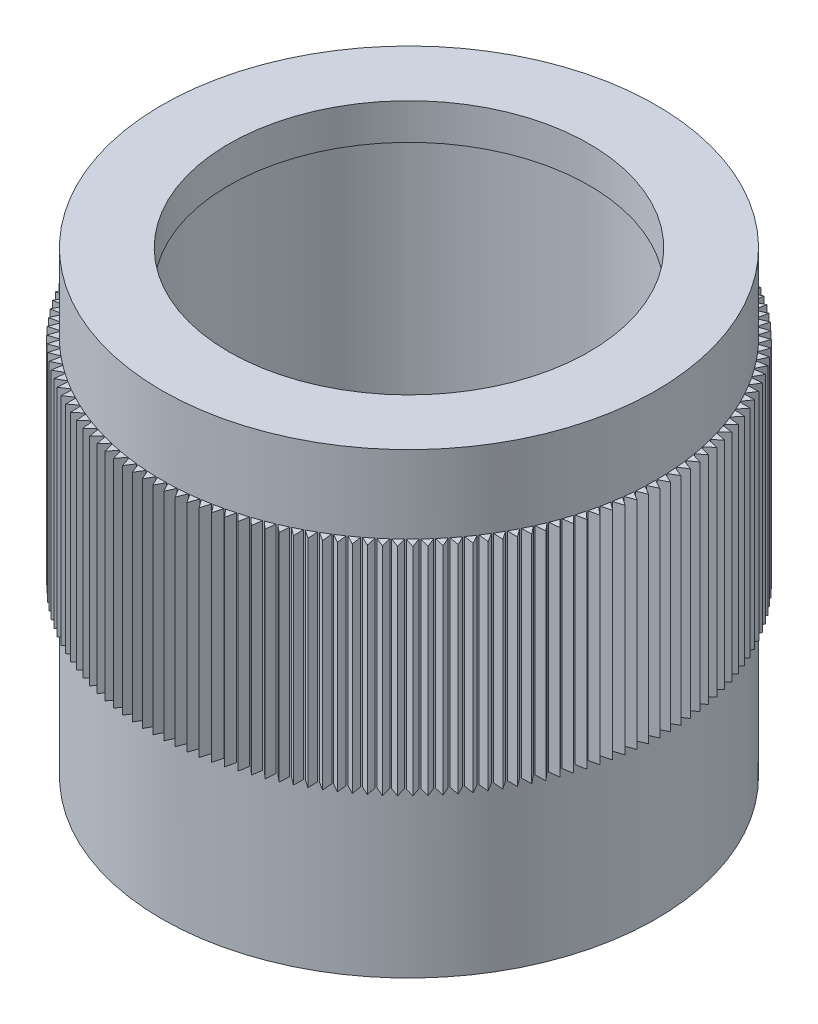
SolidWorks part; units mm, degrees
material "延性铁"
ref_plane "Front Plane" through (0, 0, 0) normal (0, 0, 1) x (1, 0, 0)
ref_plane "Top Plane" through (0, 0, 0) normal (0, 1, 0) x (1, 0, 0)
ref_plane "Right Plane" through (0, 0, 0) normal (1, 0, 0) x (0, 0, -1)
sketch "Sketch1" plane through (0, 0, 0) normal (0, 0, 1) x (1, 0, 0)
  line L0 (0, 15.2542) -> (0, -3.0391) construction
  line L1 (-5, 11.7) -> (-5.25, 11.7)
  line L2 (-5.25, 11.7) -> (-5.25, 0)
  line L3 (-5.25, 0) -> (-6.86, 0)
  line L4 (-6.86, 0) -> (-6.86, 12.7)
  line L5 (-6.86, 12.7) -> (-5, 12.7)
  line L6 (-5, 12.7) -> (-5, 11.7)
  dimension "D1" = 13.72
  dimension "D2" = 10.5
  dimension "D3" = 1
  dimension "D4" = 12.7
  dimension "D5" = 10
revolve "Revolve1" add sketch "Sketch1" angle 360 about L0
cosmetic thread "Cosmetic Thread2" parameters "D1"=8, "D2"=10.7
ref_plane "Plane1" through (0, 10.55, 0) normal (0, 1, 0) x (-1, 0, 0)
sketch "Sketch2" plane through (0, 10.55, 0) normal (0, 1, 0) x (-1, 0, 0)
  line L0 (0, -1.1989) -> (0, 9.5046) construction
  line L1 (-0.125, 6.8589) -> (0, 7.11)
  line L2 (0, 7.11) -> (0.125, 6.8589)
  line L3 (0.1623, 6.8581) -> (0.2977, 7.1038)
  line L4 (0.2977, 7.1038) -> (0.4121, 6.8476)
  line L5 (0.4494, 6.8453) -> (0.5949, 7.0851)
  line L6 (0.5949, 7.0851) -> (0.6985, 6.8243)
  line L7 (0.7356, 6.8204) -> (0.8911, 7.0539)
  line L8 (0.8911, 7.0539) -> (0.9837, 6.7891)
  line L9 (1.0206, 6.7837) -> (1.1857, 7.0104)
  line L10 (1.1857, 7.0104) -> (1.2671, 6.742)
  line L11 (1.3038, 6.735) -> (1.4783, 6.9546)
  line L12 (1.4783, 6.9546) -> (1.5483, 6.683)
  line L13 (1.5847, 6.6745) -> (1.7682, 6.8866)
  line L14 (1.7682, 6.8866) -> (1.8268, 6.6123)
  line L15 (1.8628, 6.6023) -> (2.055, 6.8065)
  line L16 (2.055, 6.8065) -> (2.1021, 6.53)
  line L17 (2.1376, 6.5185) -> (2.3382, 6.7145)
  line L18 (2.3382, 6.7145) -> (2.3737, 6.4362)
  line L19 (2.4087, 6.4232) -> (2.6174, 6.6107)
  line L20 (2.6174, 6.6107) -> (2.6411, 6.3312)
  line L21 (2.6756, 6.3167) -> (2.8919, 6.4953)
  line L22 (2.8919, 6.4953) -> (2.9039, 6.215)
  line L23 (2.9377, 6.1991) -> (3.1614, 6.3685)
  line L24 (3.1614, 6.3685) -> (3.1617, 6.088)
  line L25 (3.1947, 6.0707) -> (3.4253, 6.2305)
  line L26 (3.4253, 6.2305) -> (3.4138, 5.9502)
  line L27 (3.4462, 5.9316) -> (3.6832, 6.0816)
  line L28 (3.6832, 6.0816) -> (3.66, 5.8021)
  line L29 (3.6915, 5.7821) -> (3.9346, 5.9221)
  line L30 (3.9346, 5.9221) -> (3.8998, 5.6437)
  line L31 (3.9304, 5.6224) -> (4.1792, 5.7521)
  line L32 (4.1792, 5.7521) -> (4.1327, 5.4755)
  line L33 (4.1624, 5.4529) -> (4.4164, 5.5721)
  line L34 (4.4164, 5.5721) -> (4.3583, 5.2976)
  line L35 (4.3871, 5.2738) -> (4.6458, 5.3822)
  line L36 (4.6458, 5.3822) -> (4.5763, 5.1104)
  line L37 (4.6041, 5.0855) -> (4.8671, 5.183)
  line L38 (4.8671, 5.183) -> (4.7863, 4.9143)
  line L39 (4.813, 4.8882) -> (5.0799, 4.9746)
  line L40 (5.0799, 4.9746) -> (4.9879, 4.7096)
  line L41 (5.0135, 4.6824) -> (5.2838, 4.7575)
  line L42 (5.2838, 4.7575) -> (5.1808, 4.4966)
  line L43 (5.2052, 4.4683) -> (5.4783, 4.5321)
  line L44 (5.4783, 4.5321) -> (5.3645, 4.2757)
  line L45 (5.3877, 4.2464) -> (5.6633, 4.2987)
  line L46 (5.6633, 4.2987) -> (5.5389, 4.0473)
  line L47 (5.5608, 4.0171) -> (5.8384, 4.0578)
  line L48 (5.8384, 4.0578) -> (5.7035, 3.8118)
  line L49 (5.7241, 3.7807) -> (6.0032, 3.8097)
  line L50 (6.0032, 3.8097) -> (5.8581, 3.5696)
  line L51 (5.8774, 3.5377) -> (6.1574, 3.555)
  line L52 (6.1574, 3.555) -> (6.0024, 3.3212)
  line L53 (6.0204, 3.2885) -> (6.3009, 3.294)
  line L54 (6.3009, 3.294) -> (6.1363, 3.0669)
  line L55 (6.1529, 3.0335) -> (6.4333, 3.0273)
  line L56 (6.4333, 3.0273) -> (6.2593, 2.8073)
  line L57 (6.2745, 2.7731) -> (6.5544, 2.7552)
  line L58 (6.5544, 2.7552) -> (6.3714, 2.5427)
  line L59 (6.3851, 2.508) -> (6.6641, 2.4783)
  line L60 (6.6641, 2.4783) -> (6.4723, 2.2736)
  line L61 (6.4845, 2.2384) -> (6.762, 2.1971)
  line L62 (6.762, 2.1971) -> (6.5618, 2.0006)
  line L63 (6.5726, 1.9649) -> (6.8481, 1.912)
  line L64 (6.8481, 1.912) -> (6.6398, 1.7241)
  line L65 (6.6491, 1.6879) -> (6.9221, 1.6236)
  line L66 (6.9221, 1.6236) -> (6.7062, 1.4445)
  line L67 (6.7139, 1.408) -> (6.9841, 1.3323)
  line L68 (6.9841, 1.3323) -> (6.7608, 1.1624)
  line L69 (6.767, 1.1256) -> (7.0337, 1.0387)
  line L70 (7.0337, 1.0387) -> (6.8035, 0.8783)
  line L71 (6.8082, 0.8413) -> (7.0711, 0.7432)
  line L72 (7.0711, 0.7432) -> (6.8344, 0.5926)
  line L73 (6.8375, 0.5554) -> (7.096, 0.4464)
  line L74 (7.096, 0.4464) -> (6.8532, 0.3059)
  line L75 (6.8547, 0.2686) -> (7.1084, 0.1489)
  line L76 (7.1084, 0.1489) -> (6.86, 0.0187)
  line L77 (6.86, -0.0187) -> (7.1084, -0.1489)
  line L78 (7.1084, -0.1489) -> (6.8547, -0.2686)
  line L79 (6.8532, -0.3059) -> (7.096, -0.4464)
  line L80 (7.096, -0.4464) -> (6.8375, -0.5554)
  line L81 (6.8344, -0.5926) -> (7.0711, -0.7432)
  line L82 (7.0711, -0.7432) -> (6.8082, -0.8413)
  line L83 (6.8035, -0.8783) -> (7.0337, -1.0387)
  line L84 (7.0337, -1.0387) -> (6.767, -1.1256)
  line L85 (6.7608, -1.1624) -> (6.9841, -1.3323)
  line L86 (6.9841, -1.3323) -> (6.7139, -1.408)
  line L87 (6.7062, -1.4445) -> (6.9221, -1.6236)
  line L88 (6.9221, -1.6236) -> (6.6491, -1.6879)
  line L89 (6.6398, -1.7241) -> (6.8481, -1.912)
  line L90 (6.8481, -1.912) -> (6.5726, -1.9649)
  line L91 (6.5618, -2.0006) -> (6.762, -2.1971)
  line L92 (6.762, -2.1971) -> (6.4845, -2.2384)
  line L93 (6.4723, -2.2736) -> (6.6641, -2.4783)
  line L94 (6.6641, -2.4783) -> (6.3851, -2.508)
  line L95 (6.3714, -2.5427) -> (6.5544, -2.7552)
  line L96 (6.5544, -2.7552) -> (6.2745, -2.7731)
  line L97 (6.2593, -2.8073) -> (6.4333, -3.0273)
  line L98 (6.4333, -3.0273) -> (6.1529, -3.0335)
  line L99 (6.1363, -3.0669) -> (6.3009, -3.294)
  line L100 (6.3009, -3.294) -> (6.0204, -3.2885)
  line L101 (6.0024, -3.3212) -> (6.1574, -3.555)
  line L102 (6.1574, -3.555) -> (5.8774, -3.5377)
  line L103 (5.8581, -3.5696) -> (6.0032, -3.8097)
  line L104 (6.0032, -3.8097) -> (5.7241, -3.7807)
  line L105 (5.7035, -3.8118) -> (5.8384, -4.0578)
  line L106 (5.8384, -4.0578) -> (5.5608, -4.0171)
  line L107 (5.5389, -4.0473) -> (5.6633, -4.2987)
  line L108 (5.6633, -4.2987) -> (5.3877, -4.2464)
  line L109 (5.3645, -4.2757) -> (5.4783, -4.5321)
  line L110 (5.4783, -4.5321) -> (5.2052, -4.4683)
  line L111 (5.1808, -4.4966) -> (5.2838, -4.7575)
  line L112 (5.2838, -4.7575) -> (5.0135, -4.6824)
  line L113 (4.9879, -4.7096) -> (5.0799, -4.9746)
  line L114 (5.0799, -4.9746) -> (4.813, -4.8882)
  line L115 (4.7863, -4.9143) -> (4.8671, -5.183)
  line L116 (4.8671, -5.183) -> (4.6041, -5.0855)
  line L117 (4.5763, -5.1104) -> (4.6458, -5.3822)
  line L118 (4.6458, -5.3822) -> (4.3871, -5.2738)
  line L119 (4.3583, -5.2976) -> (4.4164, -5.5721)
  line L120 (4.4164, -5.5721) -> (4.1624, -5.4529)
  line L121 (4.1327, -5.4755) -> (4.1792, -5.7521)
  line L122 (4.1792, -5.7521) -> (3.9304, -5.6224)
  line L123 (3.8998, -5.6437) -> (3.9346, -5.9221)
  line L124 (3.9346, -5.9221) -> (3.6915, -5.7821)
  line L125 (3.66, -5.8021) -> (3.6832, -6.0816)
  line L126 (3.6832, -6.0816) -> (3.4462, -5.9316)
  line L127 (3.4138, -5.9502) -> (3.4253, -6.2305)
  line L128 (3.4253, -6.2305) -> (3.1947, -6.0707)
  line L129 (3.1617, -6.088) -> (3.1614, -6.3685)
  line L130 (3.1614, -6.3685) -> (2.9377, -6.1991)
  line L131 (2.9039, -6.215) -> (2.8919, -6.4953)
  line L132 (2.8919, -6.4953) -> (2.6756, -6.3167)
  line L133 (2.6411, -6.3312) -> (2.6174, -6.6107)
  line L134 (2.6174, -6.6107) -> (2.4087, -6.4232)
  line L135 (2.3737, -6.4362) -> (2.3382, -6.7145)
  line L136 (2.3382, -6.7145) -> (2.1376, -6.5185)
  line L137 (2.1021, -6.53) -> (2.055, -6.8065)
  line L138 (2.055, -6.8065) -> (1.8628, -6.6023)
  line L139 (1.8268, -6.6123) -> (1.7682, -6.8866)
  line L140 (1.7682, -6.8866) -> (1.5847, -6.6745)
  line L141 (1.5483, -6.683) -> (1.4783, -6.9546)
  line L142 (1.4783, -6.9546) -> (1.3038, -6.735)
  line L143 (1.2671, -6.742) -> (1.1857, -7.0104)
  line L144 (1.1857, -7.0104) -> (1.0206, -6.7837)
  line L145 (0.9837, -6.7891) -> (0.8911, -7.0539)
  line L146 (0.8911, -7.0539) -> (0.7356, -6.8204)
  line L147 (0.6985, -6.8243) -> (0.5949, -7.0851)
  line L148 (0.5949, -7.0851) -> (0.4494, -6.8453)
  line L149 (0.4121, -6.8476) -> (0.2977, -7.1038)
  line L150 (0.2977, -7.1038) -> (0.1623, -6.8581)
  line L151 (0.125, -6.8589) -> (0, -7.11)
  line L152 (0, -7.11) -> (-0.125, -6.8589)
  line L153 (-0.1623, -6.8581) -> (-0.2977, -7.1038)
  line L154 (-0.2977, -7.1038) -> (-0.4121, -6.8476)
  line L155 (-0.4494, -6.8453) -> (-0.5949, -7.0851)
  line L156 (-0.5949, -7.0851) -> (-0.6985, -6.8243)
  line L157 (-0.7356, -6.8204) -> (-0.8911, -7.0539)
  line L158 (-0.8911, -7.0539) -> (-0.9837, -6.7891)
  line L159 (-1.0206, -6.7837) -> (-1.1857, -7.0104)
  line L160 (-1.1857, -7.0104) -> (-1.2671, -6.742)
  line L161 (-1.3038, -6.735) -> (-1.4783, -6.9546)
  line L162 (-1.4783, -6.9546) -> (-1.5483, -6.683)
  line L163 (-1.5847, -6.6745) -> (-1.7682, -6.8866)
  line L164 (-1.7682, -6.8866) -> (-1.8268, -6.6123)
  line L165 (-1.8628, -6.6023) -> (-2.055, -6.8065)
  line L166 (-2.055, -6.8065) -> (-2.1021, -6.53)
  line L167 (-2.1376, -6.5185) -> (-2.3382, -6.7145)
  line L168 (-2.3382, -6.7145) -> (-2.3737, -6.4362)
  line L169 (-2.4087, -6.4232) -> (-2.6174, -6.6107)
  line L170 (-2.6174, -6.6107) -> (-2.6411, -6.3312)
  line L171 (-2.6756, -6.3167) -> (-2.8919, -6.4953)
  line L172 (-2.8919, -6.4953) -> (-2.9039, -6.215)
  line L173 (-2.9377, -6.1991) -> (-3.1614, -6.3685)
  line L174 (-3.1614, -6.3685) -> (-3.1617, -6.088)
  line L175 (-3.1947, -6.0707) -> (-3.4253, -6.2305)
  line L176 (-3.4253, -6.2305) -> (-3.4138, -5.9502)
  line L177 (-3.4462, -5.9316) -> (-3.6832, -6.0816)
  line L178 (-3.6832, -6.0816) -> (-3.66, -5.8021)
  line L179 (-3.6915, -5.7821) -> (-3.9346, -5.9221)
  line L180 (-3.9346, -5.9221) -> (-3.8998, -5.6437)
  line L181 (-3.9304, -5.6224) -> (-4.1792, -5.7521)
  line L182 (-4.1792, -5.7521) -> (-4.1327, -5.4755)
  line L183 (-4.1624, -5.4529) -> (-4.4164, -5.5721)
  line L184 (-4.4164, -5.5721) -> (-4.3583, -5.2976)
  line L185 (-4.3871, -5.2738) -> (-4.6458, -5.3822)
  line L186 (-4.6458, -5.3822) -> (-4.5763, -5.1104)
  line L187 (-4.6041, -5.0855) -> (-4.8671, -5.183)
  line L188 (-4.8671, -5.183) -> (-4.7863, -4.9143)
  line L189 (-4.813, -4.8882) -> (-5.0799, -4.9746)
  line L190 (-5.0799, -4.9746) -> (-4.9879, -4.7096)
  line L191 (-5.0135, -4.6824) -> (-5.2838, -4.7575)
  line L192 (-5.2838, -4.7575) -> (-5.1808, -4.4966)
  line L193 (-5.2052, -4.4683) -> (-5.4783, -4.5321)
  line L194 (-5.4783, -4.5321) -> (-5.3645, -4.2757)
  line L195 (-5.3877, -4.2464) -> (-5.6633, -4.2987)
  line L196 (-5.6633, -4.2987) -> (-5.5389, -4.0473)
  line L197 (-5.5608, -4.0171) -> (-5.8384, -4.0578)
  line L198 (-5.8384, -4.0578) -> (-5.7035, -3.8118)
  line L199 (-5.7241, -3.7807) -> (-6.0032, -3.8097)
  line L200 (-6.0032, -3.8097) -> (-5.8581, -3.5696)
  line L201 (-5.8774, -3.5377) -> (-6.1574, -3.555)
  line L202 (-6.1574, -3.555) -> (-6.0024, -3.3212)
  line L203 (-6.0204, -3.2885) -> (-6.3009, -3.294)
  line L204 (-6.3009, -3.294) -> (-6.1363, -3.0669)
  line L205 (-6.1529, -3.0335) -> (-6.4333, -3.0273)
  line L206 (-6.4333, -3.0273) -> (-6.2593, -2.8073)
  line L207 (-6.2745, -2.7731) -> (-6.5544, -2.7552)
  line L208 (-6.5544, -2.7552) -> (-6.3714, -2.5427)
  line L209 (-6.3851, -2.508) -> (-6.6641, -2.4783)
  line L210 (-6.6641, -2.4783) -> (-6.4723, -2.2736)
  line L211 (-6.4845, -2.2384) -> (-6.762, -2.1971)
  line L212 (-6.762, -2.1971) -> (-6.5618, -2.0006)
  line L213 (-6.5726, -1.9649) -> (-6.8481, -1.912)
  line L214 (-6.8481, -1.912) -> (-6.6398, -1.7241)
  line L215 (-6.6491, -1.6879) -> (-6.9221, -1.6236)
  line L216 (-6.9221, -1.6236) -> (-6.7062, -1.4445)
  line L217 (-6.7139, -1.408) -> (-6.9841, -1.3323)
  line L218 (-6.9841, -1.3323) -> (-6.7608, -1.1624)
  line L219 (-6.767, -1.1256) -> (-7.0337, -1.0387)
  line L220 (-7.0337, -1.0387) -> (-6.8035, -0.8783)
  line L221 (-6.8082, -0.8413) -> (-7.0711, -0.7432)
  line L222 (-7.0711, -0.7432) -> (-6.8344, -0.5926)
  line L223 (-6.8375, -0.5554) -> (-7.096, -0.4464)
  line L224 (-7.096, -0.4464) -> (-6.8532, -0.3059)
  line L225 (-6.8547, -0.2686) -> (-7.1084, -0.1489)
  line L226 (-7.1084, -0.1489) -> (-6.86, -0.0187)
  line L227 (-6.86, 0.0187) -> (-7.1084, 0.1489)
  line L228 (-7.1084, 0.1489) -> (-6.8547, 0.2686)
  line L229 (-6.8532, 0.3059) -> (-7.096, 0.4464)
  line L230 (-7.096, 0.4464) -> (-6.8375, 0.5554)
  line L231 (-6.8344, 0.5926) -> (-7.0711, 0.7432)
  line L232 (-7.0711, 0.7432) -> (-6.8082, 0.8413)
  line L233 (-6.8035, 0.8783) -> (-7.0337, 1.0387)
  line L234 (-7.0337, 1.0387) -> (-6.767, 1.1256)
  line L235 (-6.7608, 1.1624) -> (-6.9841, 1.3323)
  line L236 (-6.9841, 1.3323) -> (-6.7139, 1.408)
  line L237 (-6.7062, 1.4445) -> (-6.9221, 1.6236)
  line L238 (-6.9221, 1.6236) -> (-6.6491, 1.6879)
  line L239 (-6.6398, 1.7241) -> (-6.8481, 1.912)
  line L240 (-6.8481, 1.912) -> (-6.5726, 1.9649)
  line L241 (-6.5618, 2.0006) -> (-6.762, 2.1971)
  line L242 (-6.762, 2.1971) -> (-6.4845, 2.2384)
  line L243 (-6.4723, 2.2736) -> (-6.6641, 2.4783)
  line L244 (-6.6641, 2.4783) -> (-6.3851, 2.508)
  line L245 (-6.3714, 2.5427) -> (-6.5544, 2.7552)
  line L246 (-6.5544, 2.7552) -> (-6.2745, 2.7731)
  line L247 (-6.2593, 2.8073) -> (-6.4333, 3.0273)
  line L248 (-6.4333, 3.0273) -> (-6.1529, 3.0335)
  line L249 (-6.1363, 3.0669) -> (-6.3009, 3.294)
  line L250 (-6.3009, 3.294) -> (-6.0204, 3.2885)
  line L251 (-6.0024, 3.3212) -> (-6.1574, 3.555)
  line L252 (-6.1574, 3.555) -> (-5.8774, 3.5377)
  line L253 (-5.8581, 3.5696) -> (-6.0032, 3.8097)
  line L254 (-6.0032, 3.8097) -> (-5.7241, 3.7807)
  line L255 (-5.7035, 3.8118) -> (-5.8384, 4.0578)
  line L256 (-5.8384, 4.0578) -> (-5.5608, 4.0171)
  line L257 (-5.5389, 4.0473) -> (-5.6633, 4.2987)
  line L258 (-5.6633, 4.2987) -> (-5.3877, 4.2464)
  line L259 (-5.3645, 4.2757) -> (-5.4783, 4.5321)
  line L260 (-5.4783, 4.5321) -> (-5.2052, 4.4683)
  line L261 (-5.1808, 4.4966) -> (-5.2838, 4.7575)
  line L262 (-5.2838, 4.7575) -> (-5.0135, 4.6824)
  line L263 (-4.9879, 4.7096) -> (-5.0799, 4.9746)
  line L264 (-5.0799, 4.9746) -> (-4.813, 4.8882)
  line L265 (-4.7863, 4.9143) -> (-4.8671, 5.183)
  line L266 (-4.8671, 5.183) -> (-4.6041, 5.0855)
  line L267 (-4.5763, 5.1104) -> (-4.6458, 5.3822)
  line L268 (-4.6458, 5.3822) -> (-4.3871, 5.2738)
  line L269 (-4.3583, 5.2976) -> (-4.4164, 5.5721)
  line L270 (-4.4164, 5.5721) -> (-4.1624, 5.4529)
  line L271 (-4.1327, 5.4755) -> (-4.1792, 5.7521)
  line L272 (-4.1792, 5.7521) -> (-3.9304, 5.6224)
  line L273 (-3.8998, 5.6437) -> (-3.9346, 5.9221)
  line L274 (-3.9346, 5.9221) -> (-3.6915, 5.7821)
  line L275 (-3.66, 5.8021) -> (-3.6832, 6.0816)
  line L276 (-3.6832, 6.0816) -> (-3.4462, 5.9316)
  line L277 (-3.4138, 5.9502) -> (-3.4253, 6.2305)
  line L278 (-3.4253, 6.2305) -> (-3.1947, 6.0707)
  line L279 (-3.1617, 6.088) -> (-3.1614, 6.3685)
  line L280 (-3.1614, 6.3685) -> (-2.9377, 6.1991)
  line L281 (-2.9039, 6.215) -> (-2.8919, 6.4953)
  line L282 (-2.8919, 6.4953) -> (-2.6756, 6.3167)
  line L283 (-2.6411, 6.3312) -> (-2.6174, 6.6107)
  line L284 (-2.6174, 6.6107) -> (-2.4087, 6.4232)
  line L285 (-2.3737, 6.4362) -> (-2.3382, 6.7145)
  line L286 (-2.3382, 6.7145) -> (-2.1376, 6.5185)
  line L287 (-2.1021, 6.53) -> (-2.055, 6.8065)
  line L288 (-2.055, 6.8065) -> (-1.8628, 6.6023)
  line L289 (-1.8268, 6.6123) -> (-1.7682, 6.8866)
  line L290 (-1.7682, 6.8866) -> (-1.5847, 6.6745)
  line L291 (-1.5483, 6.683) -> (-1.4783, 6.9546)
  line L292 (-1.4783, 6.9546) -> (-1.3038, 6.735)
  line L293 (-1.2671, 6.742) -> (-1.1857, 7.0104)
  line L294 (-1.1857, 7.0104) -> (-1.0206, 6.7837)
  line L295 (-0.9837, 6.7891) -> (-0.8911, 7.0539)
  line L296 (-0.8911, 7.0539) -> (-0.7356, 6.8204)
  line L297 (-0.6985, 6.8243) -> (-0.5949, 7.0851)
  line L298 (-0.5949, 7.0851) -> (-0.4494, 6.8453)
  line L299 (-0.4121, 6.8476) -> (-0.2977, 7.1038)
  line L300 (-0.2977, 7.1038) -> (-0.1623, 6.8581)
  circle A0 centre (0, 0) radius 6.86 construction
  arc A1 (0.125, 6.8589) -> (-0.125, 6.8589) centre (0, 0) ccw
  arc A2 (0.4121, 6.8476) -> (0.1623, 6.8581) centre (0, 0) ccw
  arc A3 (0.6985, 6.8243) -> (0.4494, 6.8453) centre (0, 0) ccw
  arc A4 (0.9837, 6.7891) -> (0.7356, 6.8204) centre (0, 0) ccw
  arc A5 (1.2671, 6.742) -> (1.0206, 6.7837) centre (0, 0) ccw
  arc A6 (1.5483, 6.683) -> (1.3038, 6.735) centre (0, 0) ccw
  arc A7 (1.8268, 6.6123) -> (1.5847, 6.6745) centre (0, 0) ccw
  arc A8 (2.1021, 6.53) -> (1.8628, 6.6023) centre (0, 0) ccw
  arc A9 (2.3737, 6.4362) -> (2.1376, 6.5185) centre (0, 0) ccw
  arc A10 (2.6411, 6.3312) -> (2.4087, 6.4232) centre (0, 0) ccw
  arc A11 (2.9039, 6.215) -> (2.6756, 6.3167) centre (0, 0) ccw
  arc A12 (3.1617, 6.088) -> (2.9377, 6.1991) centre (0, 0) ccw
  arc A13 (3.4138, 5.9502) -> (3.1947, 6.0707) centre (0, 0) ccw
  arc A14 (3.66, 5.8021) -> (3.4462, 5.9316) centre (0, 0) ccw
  arc A15 (3.8998, 5.6437) -> (3.6915, 5.7821) centre (0, 0) ccw
  arc A16 (4.1327, 5.4755) -> (3.9304, 5.6224) centre (0, 0) ccw
  arc A17 (4.3583, 5.2976) -> (4.1624, 5.4529) centre (0, 0) ccw
  arc A18 (4.5763, 5.1104) -> (4.3871, 5.2738) centre (0, 0) ccw
  arc A19 (4.7863, 4.9143) -> (4.6041, 5.0855) centre (0, 0) ccw
  arc A20 (4.9879, 4.7096) -> (4.813, 4.8882) centre (0, 0) ccw
  arc A21 (5.1808, 4.4966) -> (5.0135, 4.6824) centre (0, 0) ccw
  arc A22 (5.3645, 4.2757) -> (5.2052, 4.4683) centre (0, 0) ccw
  arc A23 (5.5389, 4.0473) -> (5.3877, 4.2464) centre (0, 0) ccw
  arc A24 (5.7035, 3.8118) -> (5.5608, 4.0171) centre (0, 0) ccw
  arc A25 (5.8581, 3.5696) -> (5.7241, 3.7807) centre (0, 0) ccw
  arc A26 (6.0024, 3.3212) -> (5.8774, 3.5377) centre (0, 0) ccw
  arc A27 (6.1363, 3.0669) -> (6.0204, 3.2885) centre (0, 0) ccw
  arc A28 (6.2593, 2.8073) -> (6.1529, 3.0335) centre (0, 0) ccw
  arc A29 (6.3714, 2.5427) -> (6.2745, 2.7731) centre (0, 0) ccw
  arc A30 (6.4723, 2.2736) -> (6.3851, 2.508) centre (0, 0) ccw
  arc A31 (6.5618, 2.0006) -> (6.4845, 2.2384) centre (0, 0) ccw
  arc A32 (6.6398, 1.7241) -> (6.5726, 1.9649) centre (0, 0) ccw
  arc A33 (6.7062, 1.4445) -> (6.6491, 1.6879) centre (0, 0) ccw
  arc A34 (6.7608, 1.1624) -> (6.7139, 1.408) centre (0, 0) ccw
  arc A35 (6.8035, 0.8783) -> (6.767, 1.1256) centre (0, 0) ccw
  arc A36 (6.8344, 0.5926) -> (6.8082, 0.8413) centre (0, 0) ccw
  arc A37 (6.8532, 0.3059) -> (6.8375, 0.5554) centre (0, 0) ccw
  arc A38 (6.86, 0.0187) -> (6.8547, 0.2686) centre (0, 0) ccw
  arc A39 (6.8547, -0.2686) -> (6.86, -0.0187) centre (0, 0) ccw
  arc A40 (6.8375, -0.5554) -> (6.8532, -0.3059) centre (0, 0) ccw
  arc A41 (6.8082, -0.8413) -> (6.8344, -0.5926) centre (0, 0) ccw
  arc A42 (6.767, -1.1256) -> (6.8035, -0.8783) centre (0, 0) ccw
  arc A43 (6.7139, -1.408) -> (6.7608, -1.1624) centre (0, 0) ccw
  arc A44 (6.6491, -1.6879) -> (6.7062, -1.4445) centre (0, 0) ccw
  arc A45 (6.5726, -1.9649) -> (6.6398, -1.7241) centre (0, 0) ccw
  arc A46 (6.4845, -2.2384) -> (6.5618, -2.0006) centre (0, 0) ccw
  arc A47 (6.3851, -2.508) -> (6.4723, -2.2736) centre (0, 0) ccw
  arc A48 (6.2745, -2.7731) -> (6.3714, -2.5427) centre (0, 0) ccw
  arc A49 (6.1529, -3.0335) -> (6.2593, -2.8073) centre (0, 0) ccw
  arc A50 (6.0204, -3.2885) -> (6.1363, -3.0669) centre (0, 0) ccw
  arc A51 (5.8774, -3.5377) -> (6.0024, -3.3212) centre (0, 0) ccw
  arc A52 (5.7241, -3.7807) -> (5.8581, -3.5696) centre (0, 0) ccw
  arc A53 (5.5608, -4.0171) -> (5.7035, -3.8118) centre (0, 0) ccw
  arc A54 (5.3877, -4.2464) -> (5.5389, -4.0473) centre (0, 0) ccw
  arc A55 (5.2052, -4.4683) -> (5.3645, -4.2757) centre (0, 0) ccw
  arc A56 (5.0135, -4.6824) -> (5.1808, -4.4966) centre (0, 0) ccw
  arc A57 (4.813, -4.8882) -> (4.9879, -4.7096) centre (0, 0) ccw
  arc A58 (4.6041, -5.0855) -> (4.7863, -4.9143) centre (0, 0) ccw
  arc A59 (4.3871, -5.2738) -> (4.5763, -5.1104) centre (0, 0) ccw
  arc A60 (4.1624, -5.4529) -> (4.3583, -5.2976) centre (0, 0) ccw
  arc A61 (3.9304, -5.6224) -> (4.1327, -5.4755) centre (0, 0) ccw
  arc A62 (3.6915, -5.7821) -> (3.8998, -5.6437) centre (0, 0) ccw
  arc A63 (3.4462, -5.9316) -> (3.66, -5.8021) centre (0, 0) ccw
  arc A64 (3.1947, -6.0707) -> (3.4138, -5.9502) centre (0, 0) ccw
  arc A65 (2.9377, -6.1991) -> (3.1617, -6.088) centre (0, 0) ccw
  arc A66 (2.6756, -6.3167) -> (2.9039, -6.215) centre (0, 0) ccw
  arc A67 (2.4087, -6.4232) -> (2.6411, -6.3312) centre (0, 0) ccw
  arc A68 (2.1376, -6.5185) -> (2.3737, -6.4362) centre (0, 0) ccw
  arc A69 (1.8628, -6.6023) -> (2.1021, -6.53) centre (0, 0) ccw
  arc A70 (1.5847, -6.6745) -> (1.8268, -6.6123) centre (0, 0) ccw
  arc A71 (1.3038, -6.735) -> (1.5483, -6.683) centre (0, 0) ccw
  arc A72 (1.0206, -6.7837) -> (1.2671, -6.742) centre (0, 0) ccw
  arc A73 (0.7356, -6.8204) -> (0.9837, -6.7891) centre (0, 0) ccw
  arc A74 (0.4494, -6.8453) -> (0.6985, -6.8243) centre (0, 0) ccw
  arc A75 (0.1623, -6.8581) -> (0.4121, -6.8476) centre (0, 0) ccw
  arc A76 (-0.125, -6.8589) -> (0.125, -6.8589) centre (0, 0) ccw
  arc A77 (-0.4121, -6.8476) -> (-0.1623, -6.8581) centre (0, 0) ccw
  arc A78 (-0.6985, -6.8243) -> (-0.4494, -6.8453) centre (0, 0) ccw
  arc A79 (-0.9837, -6.7891) -> (-0.7356, -6.8204) centre (0, 0) ccw
  arc A80 (-1.2671, -6.742) -> (-1.0206, -6.7837) centre (0, 0) ccw
  arc A81 (-1.5483, -6.683) -> (-1.3038, -6.735) centre (0, 0) ccw
  arc A82 (-1.8268, -6.6123) -> (-1.5847, -6.6745) centre (0, 0) ccw
  arc A83 (-2.1021, -6.53) -> (-1.8628, -6.6023) centre (0, 0) ccw
  arc A84 (-2.3737, -6.4362) -> (-2.1376, -6.5185) centre (0, 0) ccw
  arc A85 (-2.6411, -6.3312) -> (-2.4087, -6.4232) centre (0, 0) ccw
  arc A86 (-2.9039, -6.215) -> (-2.6756, -6.3167) centre (0, 0) ccw
  arc A87 (-3.1617, -6.088) -> (-2.9377, -6.1991) centre (0, 0) ccw
  arc A88 (-3.4138, -5.9502) -> (-3.1947, -6.0707) centre (0, 0) ccw
  arc A89 (-3.66, -5.8021) -> (-3.4462, -5.9316) centre (0, 0) ccw
  arc A90 (-3.8998, -5.6437) -> (-3.6915, -5.7821) centre (0, 0) ccw
  arc A91 (-4.1327, -5.4755) -> (-3.9304, -5.6224) centre (0, 0) ccw
  arc A92 (-4.3583, -5.2976) -> (-4.1624, -5.4529) centre (0, 0) ccw
  arc A93 (-4.5763, -5.1104) -> (-4.3871, -5.2738) centre (0, 0) ccw
  arc A94 (-4.7863, -4.9143) -> (-4.6041, -5.0855) centre (0, 0) ccw
  arc A95 (-4.9879, -4.7096) -> (-4.813, -4.8882) centre (0, 0) ccw
  arc A96 (-5.1808, -4.4966) -> (-5.0135, -4.6824) centre (0, 0) ccw
  arc A97 (-5.3645, -4.2757) -> (-5.2052, -4.4683) centre (0, 0) ccw
  arc A98 (-5.5389, -4.0473) -> (-5.3877, -4.2464) centre (0, 0) ccw
  arc A99 (-5.7035, -3.8118) -> (-5.5608, -4.0171) centre (0, 0) ccw
  arc A100 (-5.8581, -3.5696) -> (-5.7241, -3.7807) centre (0, 0) ccw
  arc A101 (-6.0024, -3.3212) -> (-5.8774, -3.5377) centre (0, 0) ccw
  arc A102 (-6.1363, -3.0669) -> (-6.0204, -3.2885) centre (0, 0) ccw
  arc A103 (-6.2593, -2.8073) -> (-6.1529, -3.0335) centre (0, 0) ccw
  arc A104 (-6.3714, -2.5427) -> (-6.2745, -2.7731) centre (0, 0) ccw
  arc A105 (-6.4723, -2.2736) -> (-6.3851, -2.508) centre (0, 0) ccw
  arc A106 (-6.5618, -2.0006) -> (-6.4845, -2.2384) centre (0, 0) ccw
  arc A107 (-6.6398, -1.7241) -> (-6.5726, -1.9649) centre (0, 0) ccw
  arc A108 (-6.7062, -1.4445) -> (-6.6491, -1.6879) centre (0, 0) ccw
  arc A109 (-6.7608, -1.1624) -> (-6.7139, -1.408) centre (0, 0) ccw
  arc A110 (-6.8035, -0.8783) -> (-6.767, -1.1256) centre (0, 0) ccw
  arc A111 (-6.8344, -0.5926) -> (-6.8082, -0.8413) centre (0, 0) ccw
  arc A112 (-6.8532, -0.3059) -> (-6.8375, -0.5554) centre (0, 0) ccw
  arc A113 (-6.86, -0.0187) -> (-6.8547, -0.2686) centre (0, 0) ccw
  arc A114 (-6.8547, 0.2686) -> (-6.86, 0.0187) centre (0, 0) ccw
  arc A115 (-6.8375, 0.5554) -> (-6.8532, 0.3059) centre (0, 0) ccw
  arc A116 (-6.8082, 0.8413) -> (-6.8344, 0.5926) centre (0, 0) ccw
  arc A117 (-6.767, 1.1256) -> (-6.8035, 0.8783) centre (0, 0) ccw
  arc A118 (-6.7139, 1.408) -> (-6.7608, 1.1624) centre (0, 0) ccw
  arc A119 (-6.6491, 1.6879) -> (-6.7062, 1.4445) centre (0, 0) ccw
  arc A120 (-6.5726, 1.9649) -> (-6.6398, 1.7241) centre (0, 0) ccw
  arc A121 (-6.4845, 2.2384) -> (-6.5618, 2.0006) centre (0, 0) ccw
  arc A122 (-6.3851, 2.508) -> (-6.4723, 2.2736) centre (0, 0) ccw
  arc A123 (-6.2745, 2.7731) -> (-6.3714, 2.5427) centre (0, 0) ccw
  arc A124 (-6.1529, 3.0335) -> (-6.2593, 2.8073) centre (0, 0) ccw
  arc A125 (-6.0204, 3.2885) -> (-6.1363, 3.0669) centre (0, 0) ccw
  arc A126 (-5.8774, 3.5377) -> (-6.0024, 3.3212) centre (0, 0) ccw
  arc A127 (-5.7241, 3.7807) -> (-5.8581, 3.5696) centre (0, 0) ccw
  arc A128 (-5.5608, 4.0171) -> (-5.7035, 3.8118) centre (0, 0) ccw
  arc A129 (-5.3877, 4.2464) -> (-5.5389, 4.0473) centre (0, 0) ccw
  arc A130 (-5.2052, 4.4683) -> (-5.3645, 4.2757) centre (0, 0) ccw
  arc A131 (-5.0135, 4.6824) -> (-5.1808, 4.4966) centre (0, 0) ccw
  arc A132 (-4.813, 4.8882) -> (-4.9879, 4.7096) centre (0, 0) ccw
  arc A133 (-4.6041, 5.0855) -> (-4.7863, 4.9143) centre (0, 0) ccw
  arc A134 (-4.3871, 5.2738) -> (-4.5763, 5.1104) centre (0, 0) ccw
  arc A135 (-4.1624, 5.4529) -> (-4.3583, 5.2976) centre (0, 0) ccw
  arc A136 (-3.9304, 5.6224) -> (-4.1327, 5.4755) centre (0, 0) ccw
  arc A137 (-3.6915, 5.7821) -> (-3.8998, 5.6437) centre (0, 0) ccw
  arc A138 (-3.4462, 5.9316) -> (-3.66, 5.8021) centre (0, 0) ccw
  arc A139 (-3.1947, 6.0707) -> (-3.4138, 5.9502) centre (0, 0) ccw
  arc A140 (-2.9377, 6.1991) -> (-3.1617, 6.088) centre (0, 0) ccw
  arc A141 (-2.6756, 6.3167) -> (-2.9039, 6.215) centre (0, 0) ccw
  arc A142 (-2.4087, 6.4232) -> (-2.6411, 6.3312) centre (0, 0) ccw
  arc A143 (-2.1376, 6.5185) -> (-2.3737, 6.4362) centre (0, 0) ccw
  arc A144 (-1.8628, 6.6023) -> (-2.1021, 6.53) centre (0, 0) ccw
  arc A145 (-1.5847, 6.6745) -> (-1.8268, 6.6123) centre (0, 0) ccw
  arc A146 (-1.3038, 6.735) -> (-1.5483, 6.683) centre (0, 0) ccw
  arc A147 (-1.0206, 6.7837) -> (-1.2671, 6.742) centre (0, 0) ccw
  arc A148 (-0.7356, 6.8204) -> (-0.9837, 6.7891) centre (0, 0) ccw
  arc A149 (-0.4494, 6.8453) -> (-0.6985, 6.8243) centre (0, 0) ccw
  arc A150 (-0.1623, 6.8581) -> (-0.4121, 6.8476) centre (0, 0) ccw
  dimension "D2" = 0.25
  dimension "D1" = 0.25
  dimension "D3" = 150
extrude "Boss-Extrude1" add sketch "Sketch2" against normal blind 6
chamfer "Chamfer1" distance 0.5 angle 45 1 edges at (0, 0, 5.25)
